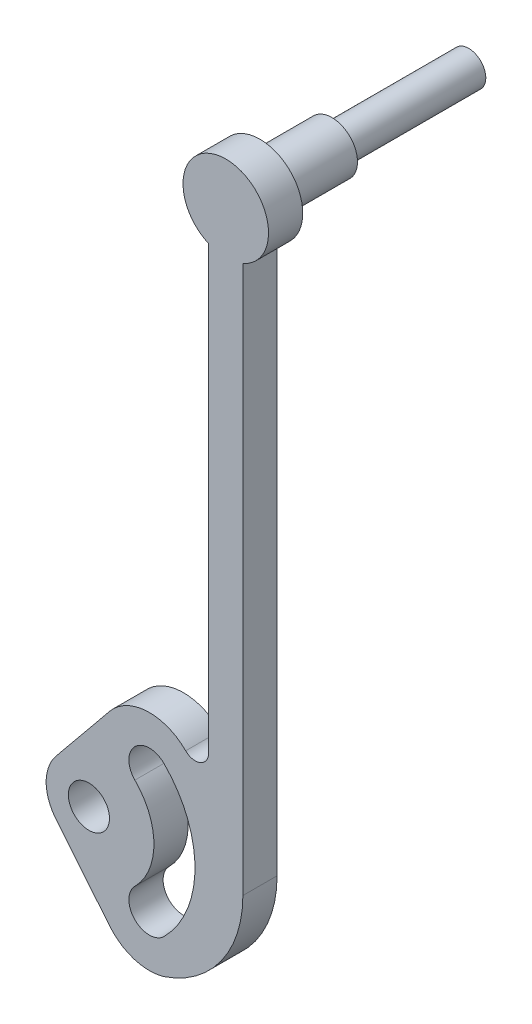
SolidWorks part; units mm, degrees
ref_plane "前视基准面" through (0, 0, 0) normal (0, 0, 1) x (1, 0, 0)
ref_plane "上视基准面" through (0, 0, 0) normal (0, 1, 0) x (1, 0, 0)
ref_plane "右视基准面" through (0, 0, 0) normal (1, 0, 0) x (0, 0, -1)
sketch "草图1" plane through (0, 0, 0) normal (0, 0, 1) x (1, 0, 0)
  line L0 (0, 0) -> (4.2426, 4.2426) construction
  line L1 (0, 0) -> (6, 0) construction
  line L2 (0, 0) -> (4.2426, -4.2426) construction
  line L3 (-9.6784, 7.9106) -> (6.0636, 27.1704)
  line L4 (-9.6784, -7.9106) -> (6.0636, -27.1704)
  line L5 (45, 0) -> (45, 160)
  line L6 (35, 160) -> (35, 31.066)
  circle A0 centre (0, 0) radius 6
  arc A1 (-9.6784, 7.9106) -> (-9.6784, -7.9106) centre (0, 0) ccw
  arc A2 (17.6777, 17.6777) -> (17.6777, -17.6777) centre (0, 0) cw construction
  arc A3 (21.9203, -21.9203) -> (21.9203, 21.9203) centre (0, 0) ccw
  arc A4 (13.435, -13.435) -> (13.435, 13.435) centre (0, 0) ccw
  arc A5 (13.435, -13.435) -> (21.9203, -21.9203) centre (17.6777, -17.6777) ccw
  arc A6 (21.9203, 21.9203) -> (13.435, 13.435) centre (17.6777, 17.6777) ccw
  arc A7 (17.6777, 17.6777) -> (17.6777, -17.6777) centre (0, 0) cw construction
  arc A8 (17.6777, 17.6777) -> (17.6777, -17.6777) centre (0, 0) cw construction
  arc A10 (45, 160) -> (35, 160) centre (40, 171.4564) ccw
  arc A11 (6.0636, -27.1704) -> (21.9203, -32.0652) centre (17.6777, -17.6777) ccw
  arc A12 (28.2843, 28.2843) -> (6.0636, 27.1704) centre (17.6777, 17.6777) ccw
  arc A13 (28.2843, 28.2843) -> (35, 31.066) centre (31.066, 31.066) ccw
  arc A14 (45, 0) -> (21.9203, -32.0652) centre (11.1857, 0) cw
  point P9 (25, 0)
  point P17 (25, 0)
  point P19 (25, 0)
  dimension "D1" = 45
  dimension "D3" = 25
  dimension "D2" = 45
extrude "凸台-拉伸1" add sketch "草图1" along normal blind 10
sketch "草图3" plane through (0, 0, 0) normal (0, 0, -1) x (-1, 0, 0)
  circle A0 centre (-40, 171.4564) radius 7.5
extrude "凸台-拉伸2" add sketch "草图3" along normal blind 21
sketch "草图4" plane through (0, 0, -21) normal (0, 0, -1) x (-1, 0, 0)
  circle A0 centre (-40, 171.4564) radius 5
extrude "凸台-拉伸3" add sketch "草图4" along normal blind 40
